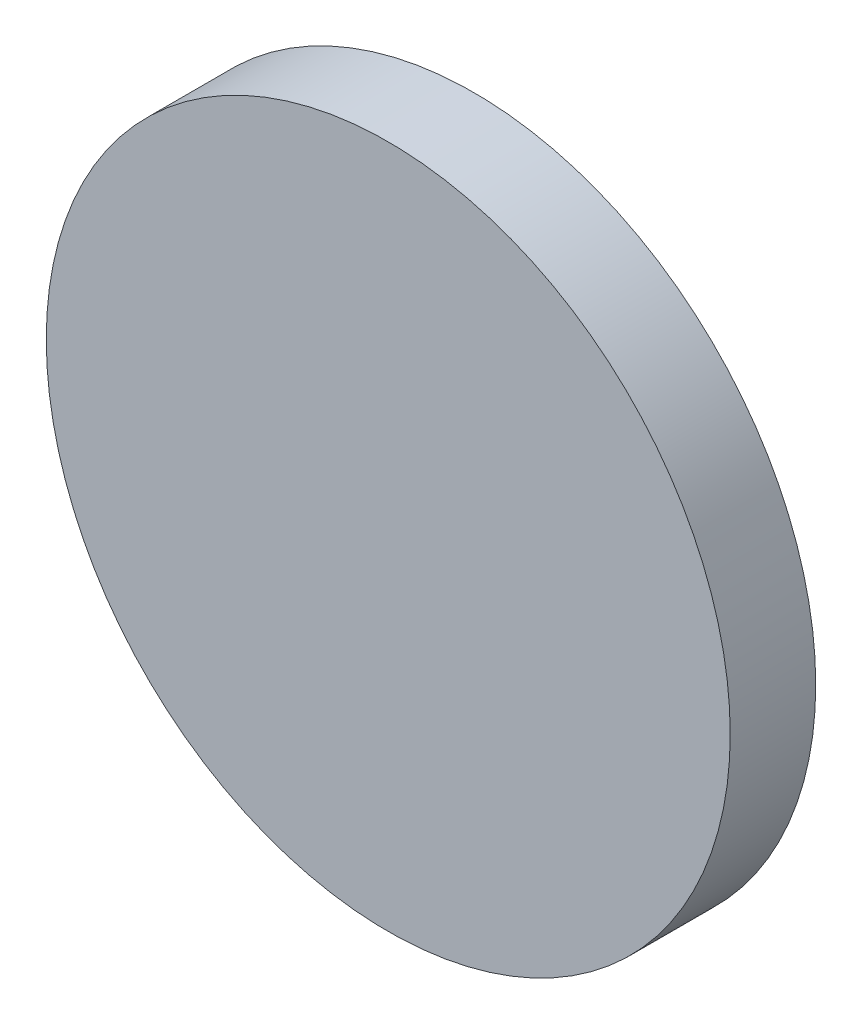
from build123d import *

# Parameters (mm, degrees)
SKETCH1_R           = 30
BOSS_EXTRUDE1_DEPTH = 7.5


with BuildPart() as part:
    # Sketch1 → Boss-Extrude1 (new body)
    with BuildSketch(Plane.XY):
        Circle(SKETCH1_R)
    extrude(amount=BOSS_EXTRUDE1_DEPTH)


solid = part.part
